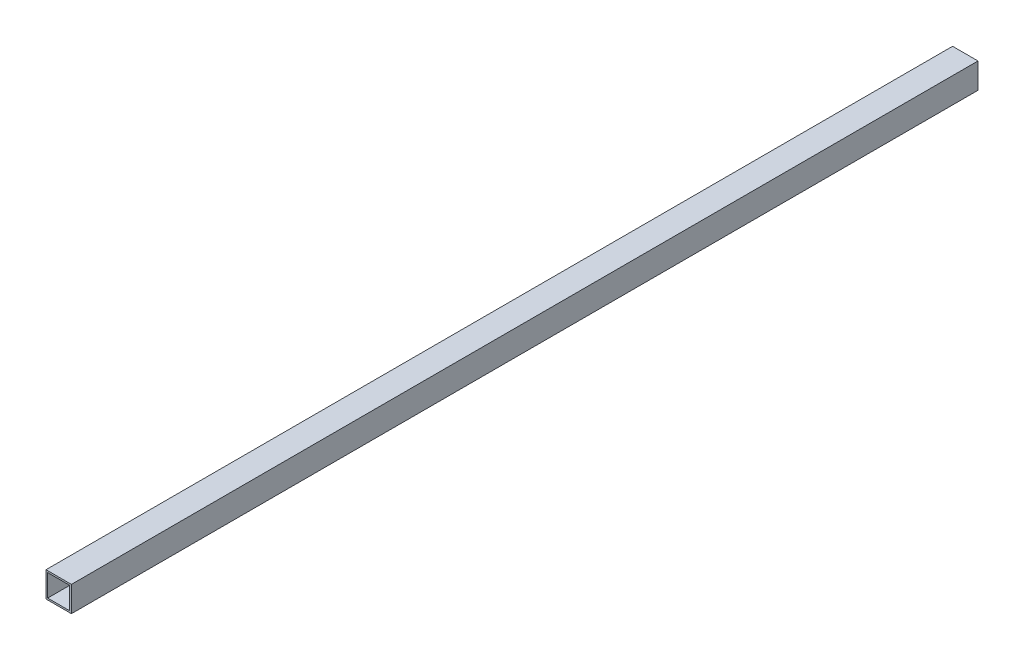
from build123d import *

# Parameters (mm, degrees)
SKETCH_1_W      = 30
SKETCH_1_H      = 30
SKETCH_1_W_2    = 26
SKETCH_1_H_2    = 26
EXTRUDE_1_DEPTH = 1070


with BuildPart() as part:
    # 草图1 → 凸台-拉伸1 (new body)
    with BuildSketch(Plane.XY):
        Rectangle(SKETCH_1_W, SKETCH_1_H)
        Rectangle(SKETCH_1_W_2, SKETCH_1_H_2, mode=Mode.SUBTRACT)
    extrude(amount=EXTRUDE_1_DEPTH)


solid = part.part
